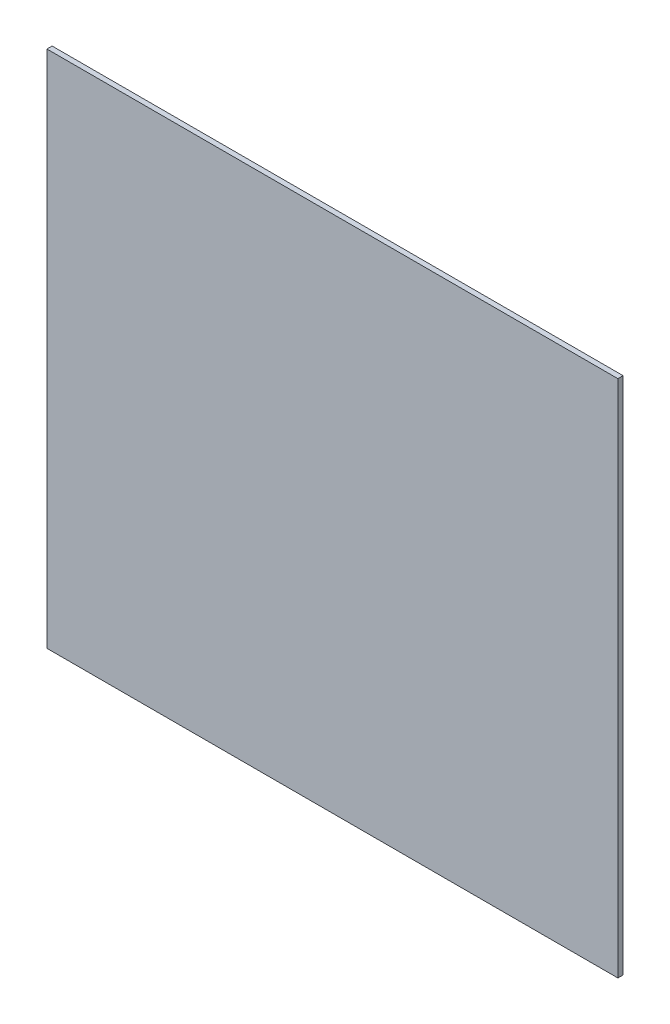
SolidWorks part; units mm, degrees
ref_plane "Front Plane" through (0, 0, 0) normal (0, 0, 1) x (1, 0, 0)
ref_plane "Top Plane" through (0, 0, 0) normal (0, 1, 0) x (1, 0, 0)
ref_plane "Right Plane" through (0, 0, 0) normal (1, 0, 0) x (0, 0, -1)
other "Configuration Table"
sketch "Sketch1" plane through (0, 0, 0) normal (0, 0, 1) x (1, 0, 0)
  line L0 (-123.6802, -124) -> (-123.6802, 121) construction
  line L1 (96.3198, -91) -> (-123.6802, -91)
  line L2 (96.3198, -91) -> (96.3198, 109)
  line L3 (96.3198, 109) -> (-123.6802, 109)
  line L4 (-123.6802, -91) -> (-123.6802, 109)
  line L5 (-114.6802, 109) -> (-121.6802, 109) construction
  dimension "D1" = 200
  dimension "D2" = 220
extrude "Boss-Extrude1" add sketch "Sketch1" along normal blind 2 contours L1 L4 L3 L2
